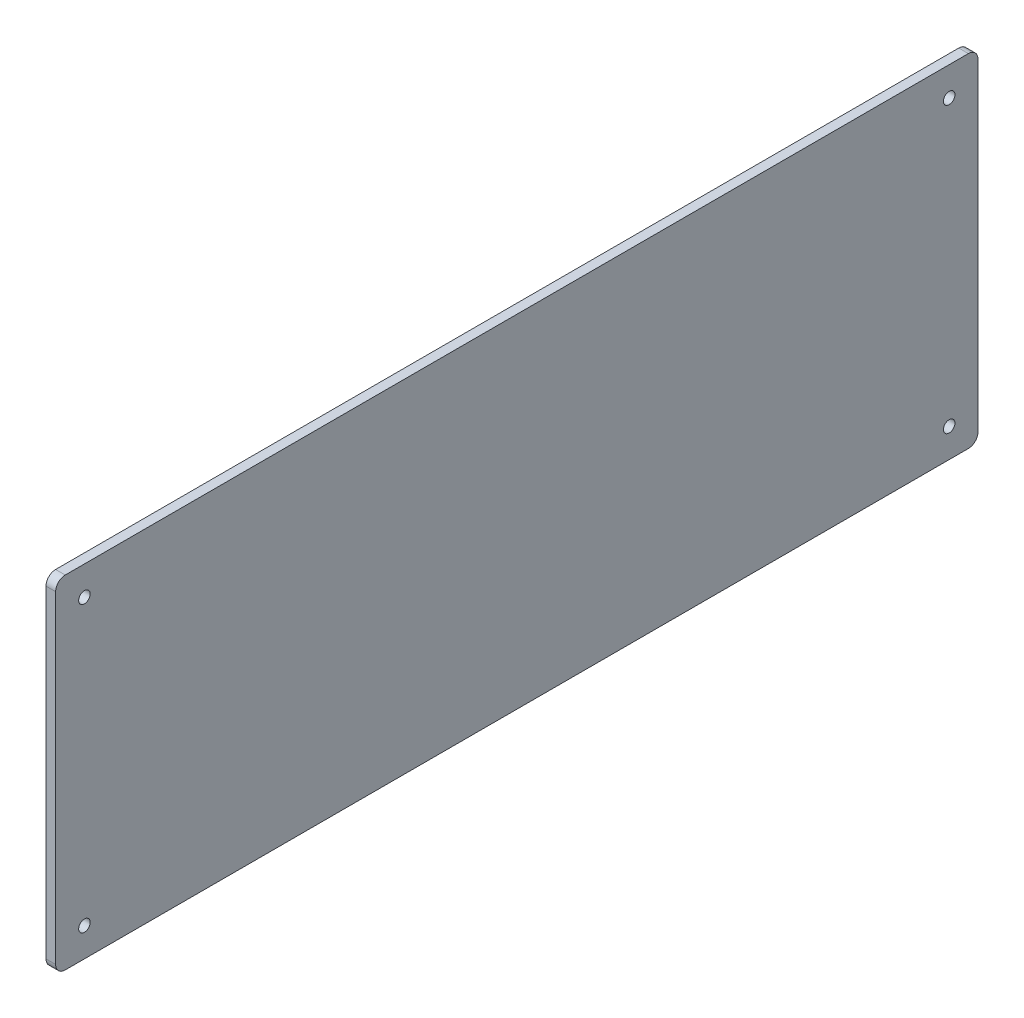
from build123d import *

# Parameters (mm, degrees)
SKETCH_1_W          = 480
SKETCH_1_H          = 178
EXTRUDE_1_DEPTH     = 5
SKETCH_2_R          = 3
CUT_EXTRUDE_1_DEPTH = 257.019530505
FILLET_1_R          = 5


with BuildPart() as part:
    # 草图1 → 凸台-拉伸1 (new body)
    with BuildSketch(Plane(origin=(0, 0, 0), x_dir=(0, 0, -1), z_dir=(1, 0, 0))):
        Rectangle(SKETCH_1_W, SKETCH_1_H)
    extrude(amount=EXTRUDE_1_DEPTH)

    # 草图2 → 切除-拉伸1 (cut, through all)
    with BuildSketch(Plane(origin=(5, 0, 0), x_dir=(0, 0, -1), z_dir=(1, 0, 0))):
        with Locations((-225, 74)):
            Circle(SKETCH_2_R)
        with Locations((225, 74)):
            Circle(SKETCH_2_R)
        with Locations((-225, -74)):
            Circle(SKETCH_2_R)
        with Locations((225, -74)):
            Circle(SKETCH_2_R)
    extrude(amount=-CUT_EXTRUDE_1_DEPTH, mode=Mode.SUBTRACT)

    # 圆角1
    fillet_1_edges = [part.edges().sort_by_distance(p)[0] for p in [
        (2.5, 89, 240),
        (2.5, 89, -240),
        (2.5, -89, -240),
        (2.5, -89, 240),
    ]]
    fillet(fillet_1_edges, radius=FILLET_1_R)


solid = part.part
